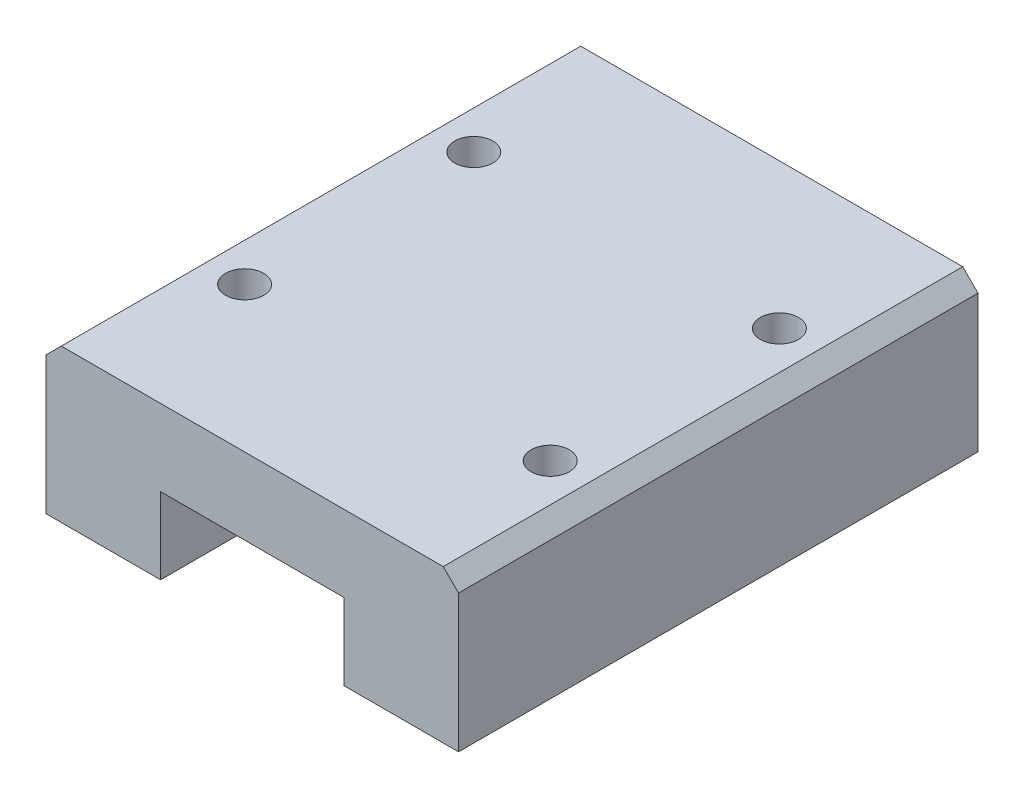
from build123d import *

# Parameters (mm, degrees)
EXTRUDE_1_DEPTH        = 34
HOLE_WIZARD_M3_1_D     = 2.5
HOLE_WIZARD_M3_1_DEPTH = 7.5
HOLE_WIZARD_M3_1_TIP   = 0.751075774
CHAMFER_1_SIZE         = 1


with BuildPart() as part:
    # 草图1 → 凸台-拉伸1 (new body)
    with BuildSketch(Plane.XY):
        Polygon((-6, 0), (6, 0), (6, -5), (13.5, -5), (13.5, 5), (-13.5, 5), (-13.5, -5), (-6, -5), align=None)
    extrude(amount=EXTRUDE_1_DEPTH)

    # M3 螺纹孔1
    with Locations(Plane(origin=(0, 5, 0), x_dir=(1, 0, 0), z_dir=(0, 1, 0))):
        with Locations((-10, -9.5), (10, -9.5), (-10, -24.5), (10, -24.5)):
            Hole(HOLE_WIZARD_M3_1_D / 2, depth=HOLE_WIZARD_M3_1_DEPTH)
            with Locations((0, 0, -(HOLE_WIZARD_M3_1_DEPTH + HOLE_WIZARD_M3_1_TIP / 2))):  # 118° drill point
                Cone(0, HOLE_WIZARD_M3_1_D / 2, HOLE_WIZARD_M3_1_TIP, mode=Mode.SUBTRACT)

    # 倒角1
    chamfer_1_edges = [part.edges().sort_by_distance(p)[0] for p in [
        (-13.5, 5, 17),
        (13.5, 5, 17),
    ]]
    chamfer(chamfer_1_edges, length=CHAMFER_1_SIZE)


solid = part.part
